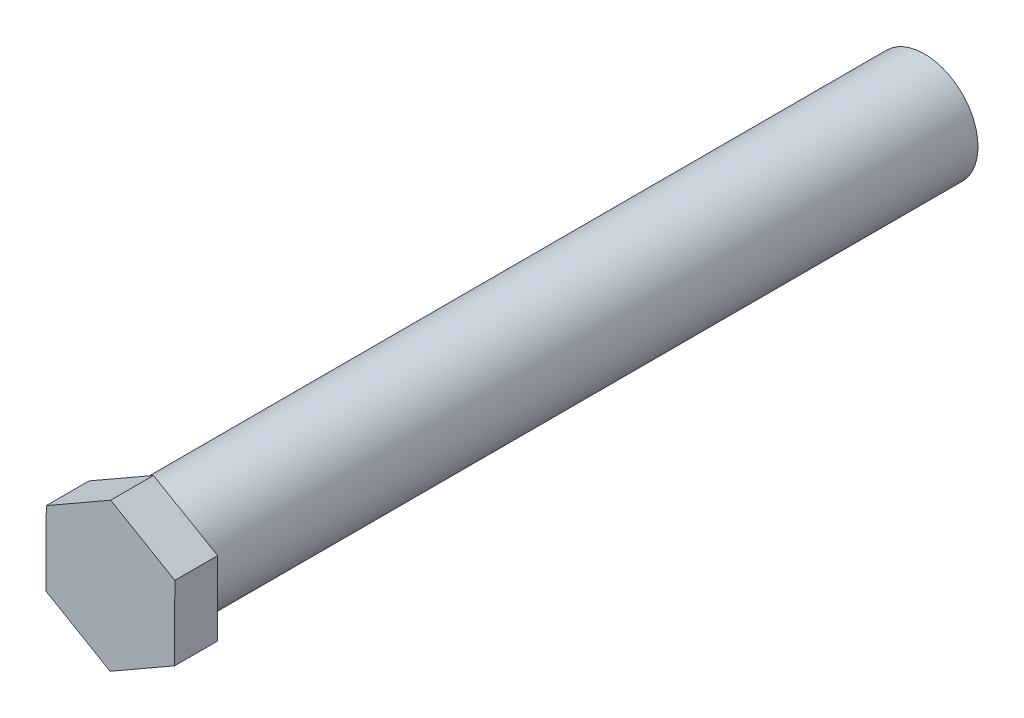
from build123d import *

# Parameters (mm, degrees)
SKETCH_1_R      = 5
EXTRUDE_1_DEPTH = 72
EXTRUDE_2_DEPTH = 4


with BuildPart() as part:
    # 草图1 → 凸台-拉伸1 (new body)
    with BuildSketch(Plane.XY):
        Circle(SKETCH_1_R)
    extrude(amount=EXTRUDE_1_DEPTH)

    # 草图2 → 凸台-拉伸2 (add)
    with BuildSketch(Plane.XY.offset(72)):
        Polygon((5.987217074, -3.486148549), (6.012701742, 3.44200781), (0.025484667, 6.928156359), (-5.987217074, 3.486148549), (-6.012701742, -3.44200781), (-0.025484667, -6.928156359), align=None)
    extrude(amount=EXTRUDE_2_DEPTH)


solid = part.part
